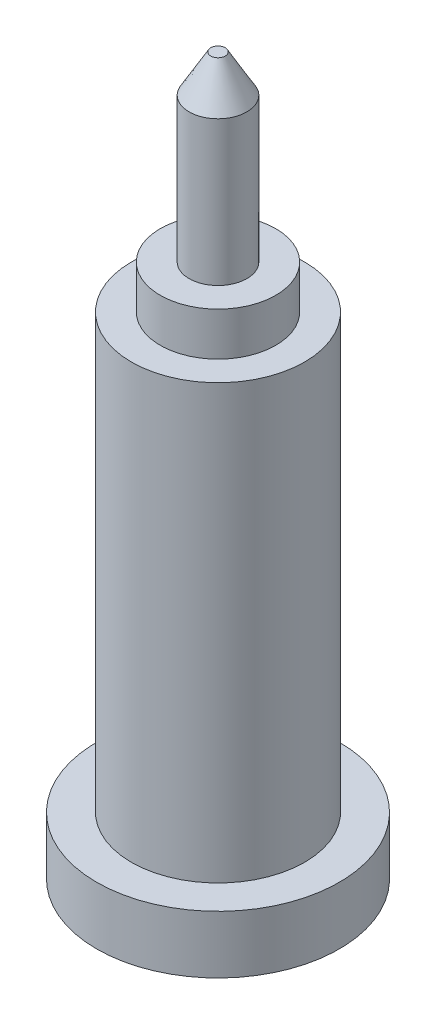
from build123d import *


with BuildPart() as part:
    # Sketch1 → Revolve1 (revolve)
    with BuildSketch(Plane.XY, mode=Mode.PRIVATE) as revolve1_sk:
        Polygon((-1.25, 0), (-4.2, 0), (-4.2, 2), (-3, 2), (-3, 17), (-2, 17), (-2, 18.5), (-1, 18.5), (-1, 23.5), (-0.25, 24.799038106), (0, 24.799038106), (0, 6), (-1.25, 6), align=None)
    revolve(revolve1_sk.sketch.rotate(Axis((0, 0, 0), (0, 1, 0)), 270), axis=Axis((0, 0, 0), (0, 1, 0)))


solid = part.part
